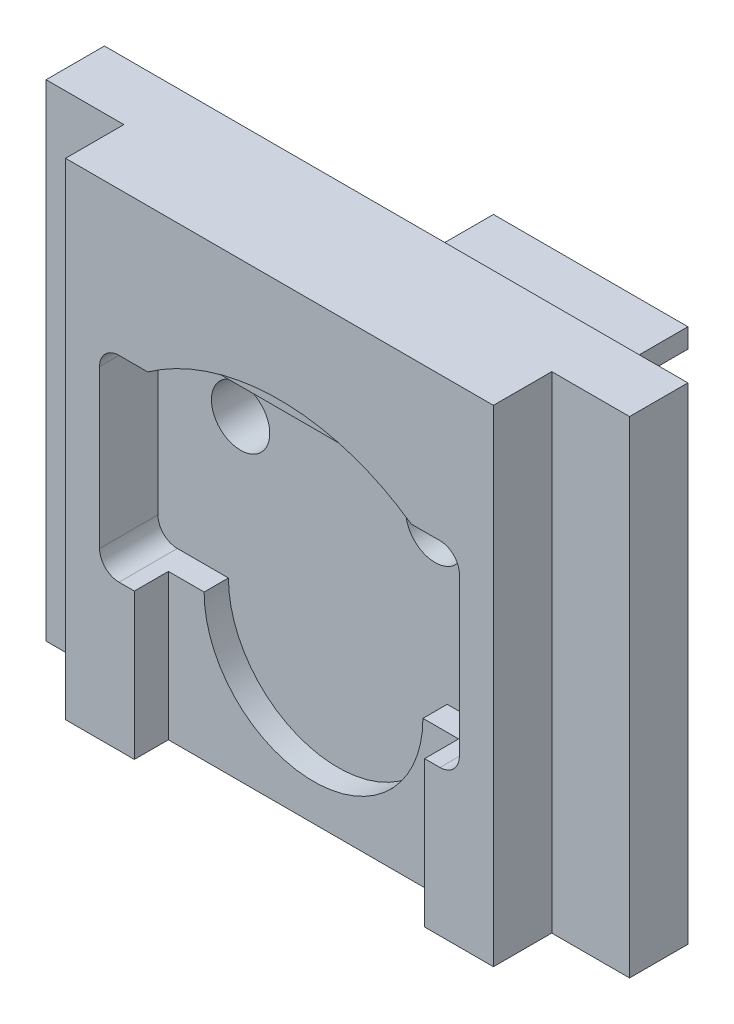
from build123d import *

# Parameters (mm, degrees)
SKETCH_1_W                      = 60
SKETCH_1_H                      = 50
EXTRUDE_1_DEPTH                 = 12
SKETCH_2_W                      = 20
SKETCH_2_H                      = 20
EXTRUDE_2_DEPTH                 = 20
SKETCH_3_R                      = 10.5
CUT_EXTRUDE_1_DEPTH             = 6
CUT_EXTRUDE_2_DEPTH             = 3.5
CUT_EXTRUDE_3_DEPTH             = 3.5
CUT_EXTRUDE_4_DEPTH             = 2.5
CUT_EXTRUDE_5_REACH             = 48.915
SKETCH_8_R                      = 3
CUT_EXTRUDE_5_DIRECTION_2_DEPTH = 47.914816423
SKETCH_9_W                      = 8
SKETCH_9_H                      = 50
CUT_EXTRUDE_6_DEPTH             = 6
CUT_EXTRUDE_START               = -2.5
SKETCH_10_W                     = 14.56297708
SKETCH_10_H                     = 20.2
CUT_EXTRUDE_7_DEPTH             = 12.5
FILLET_1_R                      = 2


with BuildPart() as part:
    # 草图1 → 凸台-拉伸1 (new body)
    with BuildSketch(Plane.XY):
        Rectangle(SKETCH_1_W, SKETCH_1_H)
    extrude(amount=EXTRUDE_1_DEPTH)

    # 草图2 → 凸台-拉伸2 (add)
    with BuildSketch(Plane(origin=(0, 0, 0), x_dir=(-1, 0, 0), z_dir=(0, 0, -1))):
        Rectangle(SKETCH_2_W, SKETCH_2_H)
    extrude(amount=EXTRUDE_2_DEPTH)

    # 草图3 → 切除-拉伸1 (cut)
    with BuildSketch(Plane.XY.offset(12)):
        with Locations((0, -10)):
            Circle(SKETCH_3_R)
    extrude(amount=-CUT_EXTRUDE_1_DEPTH, mode=Mode.SUBTRACT)

    # 草图5 → 切除-拉伸2 (cut)
    with BuildSketch(Plane.XY.offset(12)):
        with BuildLine():
            Line((-18.5, 4.964240044), (-18.5, -1.5))
            ThreePointArc((-18.5, -1.5), (-18.060660172, -2.560660172), (-17, -3))
            Line((-17, -3), (-12.845232579, -3))
            ThreePointArc((-12.845232579, -3), (-12.301125391, -2.897836674), (-11.83113527, -2.605263158))
            ThreePointArc((-11.83113527, -2.605263158), (0, 2), (11.83113527, -2.605263158))
            ThreePointArc((11.83113527, -2.605263158), (12.301125391, -2.897836674), (12.845232579, -3))
            Line((12.845232579, -3), (17, -3))
            ThreePointArc((17, -3), (18.060660172, -2.560660172), (18.5, -1.5))
            Line((18.5, -1.5), (18.5, 4.964240044))
            ThreePointArc((18.5, 4.964240044), (18.412203308, 5.469889941), (18.159090909, 5.916347319))
            ThreePointArc((18.159090909, 5.916347319), (0, 14.5), (-18.159090909, 5.916347319))
            ThreePointArc((-18.159090909, 5.916347319), (-18.412203308, 5.469889941), (-18.5, 4.964240044))
        make_face()
    extrude(amount=-CUT_EXTRUDE_2_DEPTH, mode=Mode.SUBTRACT)

    # 草图6 → 切除-拉伸3 (cut)
    with BuildSketch(Plane.XY.offset(12)):
        with BuildLine():
            Line((-13.389251051, -3), (-14.922616289, -3))
            Line((-14.922616289, -3), (-14.922616289, -25))
            Line((-14.922616289, -25), (14.922616289, -25))
            Line((14.922616289, -25), (14.922616289, -3))
            Line((14.922616289, -3), (13.389251051, -3))
            Line((13.389251051, -3), (13.389251051, -8.470382759))
            Line((13.389251051, -8.470382759), (10.387986864, -8.470382759))
            ThreePointArc((10.387986864, -8.470382759), (10.471959274, -9.233143454), (10.5, -10))
            ThreePointArc((10.5, -10), (-0.766856546, -20.471959274), (-10.387986864, -8.470382759))
            Line((-10.387986864, -8.470382759), (-13.389251051, -8.470382759))
            Line((-13.389251051, -8.470382759), (-13.389251051, -3))
        make_face()
        with BuildLine():
            Line((7.826237921, -3), (-7.826237921, -3))
            ThreePointArc((-7.826237921, -3), (-9.508983543, -5.546997419), (-10.387986864, -8.470382759))
            Line((-10.387986864, -8.470382759), (10.387986864, -8.470382759))
            ThreePointArc((10.387986864, -8.470382759), (9.508983543, -5.546997419), (7.826237921, -3))
        make_face()
        with BuildLine():
            ThreePointArc((7.826237921, -3), (0, 0.5), (-7.826237921, -3))
            Line((-7.826237921, -3), (7.826237921, -3))
        make_face()
        with BuildLine():
            ThreePointArc((-11.83113527, -2.605263158), (-12.301125391, -2.897836674), (-12.845232579, -3))
            Line((-12.845232579, -3), (-7.826237921, -3))
            ThreePointArc((-7.826237921, -3), (0, 0.5), (7.826237921, -3))
            Line((7.826237921, -3), (12.845232579, -3))
            ThreePointArc((12.845232579, -3), (12.301125391, -2.897836674), (11.83113527, -2.605263158))
            ThreePointArc((11.83113527, -2.605263158), (0, 2), (-11.83113527, -2.605263158))
        make_face()
        with BuildLine():
            Line((-12.845232579, -3), (-13.389251051, -3))
            Line((-13.389251051, -3), (-13.389251051, -8.470382759))
            Line((-13.389251051, -8.470382759), (-10.387986864, -8.470382759))
            ThreePointArc((-10.387986864, -8.470382759), (-9.508983543, -5.546997419), (-7.826237921, -3))
            Line((-7.826237921, -3), (-12.845232579, -3))
        make_face()
        with BuildLine():
            Line((12.845232579, -3), (7.826237921, -3))
            ThreePointArc((7.826237921, -3), (9.508983543, -5.546997419), (10.387986864, -8.470382759))
            Line((10.387986864, -8.470382759), (13.389251051, -8.470382759))
            Line((13.389251051, -8.470382759), (13.389251051, -3))
            Line((13.389251051, -3), (12.845232579, -3))
        make_face()
    extrude(amount=-CUT_EXTRUDE_3_DEPTH, mode=Mode.SUBTRACT)

    # 草图7 → 切除-拉伸4 (cut)
    with BuildSketch(Plane.XY.offset(8.5)):
        with BuildLine():
            Line((-18.5, 0.049973913), (-18.5, 0))
            ThreePointArc((-18.5, 0), (-18.060660172, -1.060660172), (-17, -1.5))
            Line((-17, -1.5), (-12.371843032, -1.5))
            ThreePointArc((-12.371843032, -1.5), (-10.253202816, -2.672836244), (-10.122417026, -5.090909091))
            ThreePointArc((-10.122417026, -5.090909091), (0, -21.25), (10.122417026, -5.090909091))
            ThreePointArc((10.122417026, -5.090909091), (10.253202816, -2.672836244), (12.371843032, -1.5))
            Line((12.371843032, -1.5), (17, -1.5))
            ThreePointArc((17, -1.5), (18.060660172, -1.060660172), (18.5, 0))
            Line((18.5, 0), (18.5, 0.049973913))
            ThreePointArc((18.5, 0.049973913), (18.340320328, 0.929121661), (17.881679389, 1.69596379))
            ThreePointArc((17.881679389, 1.69596379), (12.348306903, 6.580233667), (5.752265423, 9.891810345))
            ThreePointArc((5.752265423, 9.891810345), (4.857632257, 10.122405227), (3.93702292, 10.2))
            Line((3.93702292, 10.2), (-3.93702292, 10.2))
            ThreePointArc((-3.93702292, 10.2), (-4.857632257, 10.122405227), (-5.752265423, 9.891810345))
            ThreePointArc((-5.752265423, 9.891810345), (-12.348306903, 6.580233667), (-17.881679389, 1.69596379))
            ThreePointArc((-17.881679389, 1.69596379), (-18.340320328, 0.929121661), (-18.5, 0.049973913))
        make_face()
    extrude(amount=-CUT_EXTRUDE_4_DEPTH, mode=Mode.SUBTRACT)

    # 草图8 → 切除-拉伸5 (cut, up to next)
    with BuildSketch(Plane.XY.offset(6), mode=Mode.PRIVATE) as cut_extrude_5_sk1:
        with Locations(Location((-10, 5, 0), (0, 0, 153.145976086))):
            Circle(SKETCH_8_R)
    cut_extrude_5_tool1 = extrude(cut_extrude_5_sk1.sketch, amount=-CUT_EXTRUDE_5_REACH, mode=Mode.PRIVATE) & part.part
    # 草图8 → 切除-拉伸5 (cut, up to next)
    with BuildSketch(Plane.XY.offset(6), mode=Mode.PRIVATE) as cut_extrude_5_sk2:
        with Locations(Location((10, 5, 0), (0, 0, 90))):
            Circle(SKETCH_8_R)
    cut_extrude_5_tool2 = extrude(cut_extrude_5_sk2.sketch, amount=-CUT_EXTRUDE_5_REACH, mode=Mode.PRIVATE) & part.part
    add(cut_extrude_5_tool1.solids().sort_by_distance((-10, 5, 6))[0], mode=Mode.SUBTRACT)
    add(cut_extrude_5_tool2.solids().sort_by_distance((10, 5, 6))[0], mode=Mode.SUBTRACT)

    # 草图8 → 切除-拉伸5 direction 2 (cut)
    with BuildSketch(Plane.XY.offset(6)):
        with Locations(Location((-10, 5, 0), (0, 0, 153.145976086))):
            Circle(SKETCH_8_R)
        with Locations(Location((10, 5, 0), (0, 0, 90))):
            Circle(SKETCH_8_R)
    extrude(amount=CUT_EXTRUDE_5_DIRECTION_2_DEPTH, mode=Mode.SUBTRACT)

    # 草图9 → 切除-拉伸6 (cut)
    with BuildSketch(Plane.XY.offset(12)):
        with Locations((-26, 0)):
            Rectangle(SKETCH_9_W, SKETCH_9_H)
        with Locations((26, 0)):
            Rectangle(SKETCH_9_W, SKETCH_9_H)
    extrude(amount=-CUT_EXTRUDE_6_DEPTH, mode=Mode.SUBTRACT)

    # 草图10 → 切除-拉伸7 (cut)
    with BuildSketch(Plane.XY.offset(8.5).offset(CUT_EXTRUDE_START)):
        with Locations((-11.21851146, 0.1)):
            Rectangle(SKETCH_10_W, SKETCH_10_H)
    cut_extrude_7 = extrude(amount=CUT_EXTRUDE_7_DEPTH, mode=Mode.SUBTRACT)

    # 镜向2: 切除-拉伸7 across plane
    add(cut_extrude_7.mirror(Plane(origin=(0, 0, 0), x_dir=(0, 0, 1), z_dir=(1, 0, 0))), mode=Mode.SUBTRACT)

    # 圆角1
    fillet_1_edges = [part.edges().sort_by_distance(p)[0] for p in [
        (-18.5, 10.2, 9),
        (-18.5, -10, 9),
        (18.5, -10, 9),
        (18.5, 10.2, 9),
    ]]
    fillet(fillet_1_edges, radius=FILLET_1_R)


solid = part.part
